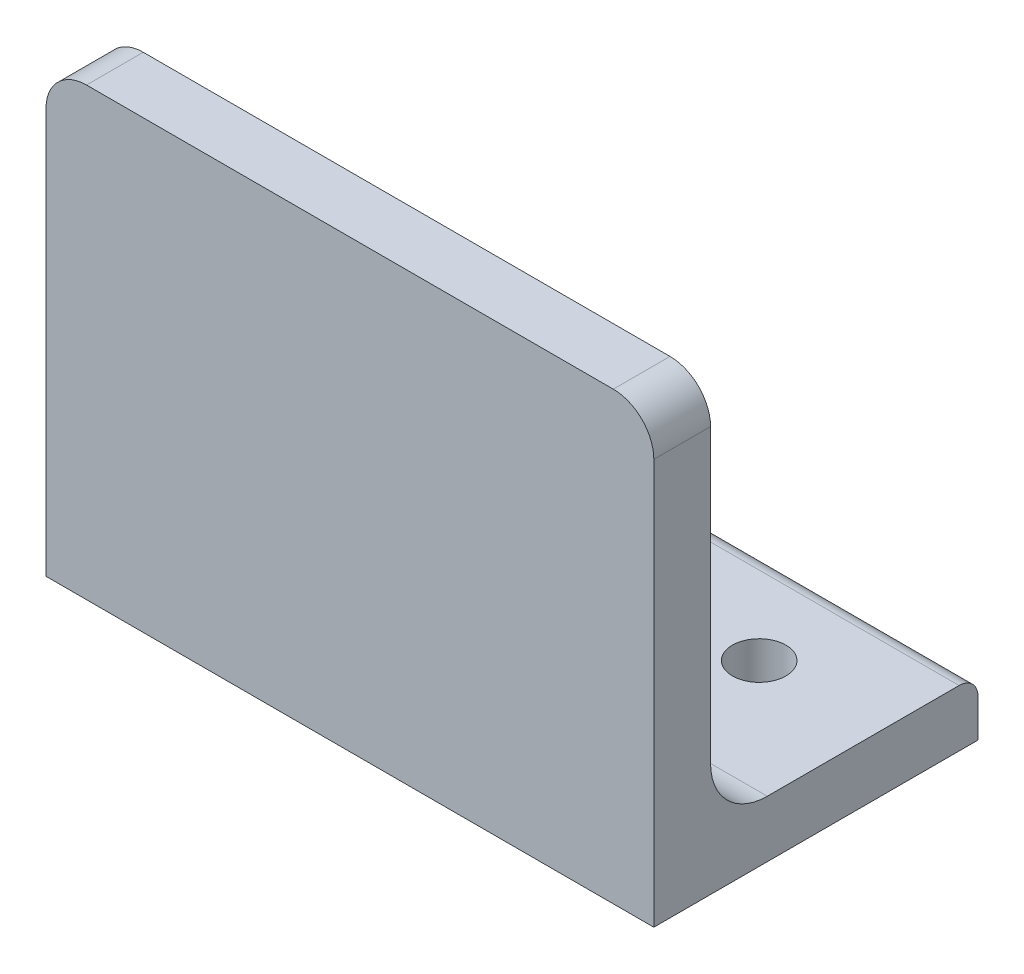
from build123d import *

# Parameters (mm, degrees)
UNEQUAL_ANGLE_6_3_4_1_DEPTH = 75
M6_CLEARANCE_HOLE1_D        = 6.6
M6_CLEARANCE_HOLE1_DEPTH    = 20
M6_CLEARANCE_HOLE1_TIP      = 1.982840043
CUT_EXTRUDE1_DEPTH          = 106.80170131
CUT_EXTRUDE1_DEPTH_BACK     = 106.80170131
SKETCH8_W                   = 14
SKETCH8_H                   = 16
FILLET1_R                   = 5


with BuildPart() as part:
    # Sketch11 → Unequal angle 6.3-4(1) (new body)
    with BuildSketch(Plane.YZ):
        with BuildLine():
            Line((63, 0), (0, 0))
            Line((0, 0), (0, -40))
            Line((0, -40), (4.666666667, -40))
            ThreePointArc((4.666666667, -40), (6.316582489, -39.316582489), (7, -37.666666667))
            Line((7, -37.666666667), (7, -14))
            ThreePointArc((7, -14), (9.050252532, -9.050252532), (14, -7))
            Line((14, -7), (60.666666667, -7))
            ThreePointArc((60.666666667, -7), (62.316582489, -6.316582489), (63, -4.666666667))
            Line((63, -4.666666667), (63, 0))
        make_face()
    extrude(amount=UNEQUAL_ANGLE_6_3_4_1_DEPTH)

    # M6 Clearance Hole1
    with Locations(Plane.XZ):
        with Locations((15, -28), (60, -28)):
            Hole(M6_CLEARANCE_HOLE1_D / 2, depth=M6_CLEARANCE_HOLE1_DEPTH)
            with Locations((0, 0, -(M6_CLEARANCE_HOLE1_DEPTH + M6_CLEARANCE_HOLE1_TIP / 2))):  # 118° drill point
                Cone(0, M6_CLEARANCE_HOLE1_D / 2, M6_CLEARANCE_HOLE1_TIP, mode=Mode.SUBTRACT)

    # Sketch8 → Cut-Extrude1 (cut, two sides: drawn at the far end of the back side and taken through both)
    with BuildSketch(Plane(origin=(75, 0, 0), x_dir=(0, 0, -1), z_dir=(1, 0, 0)).offset(-CUT_EXTRUDE1_DEPTH_BACK)):
        with Locations((0, 63)):
            Rectangle(SKETCH8_W, SKETCH8_H)
    extrude(amount=CUT_EXTRUDE1_DEPTH + CUT_EXTRUDE1_DEPTH_BACK, mode=Mode.SUBTRACT)

    # Fillet1
    fillet1_edges = [part.edges().sort_by_distance(p)[0] for p in [
        (0, 55, -3.5),
        (75, 55, -3.5),
    ]]
    fillet(fillet1_edges, radius=FILLET1_R)


solid = part.part
